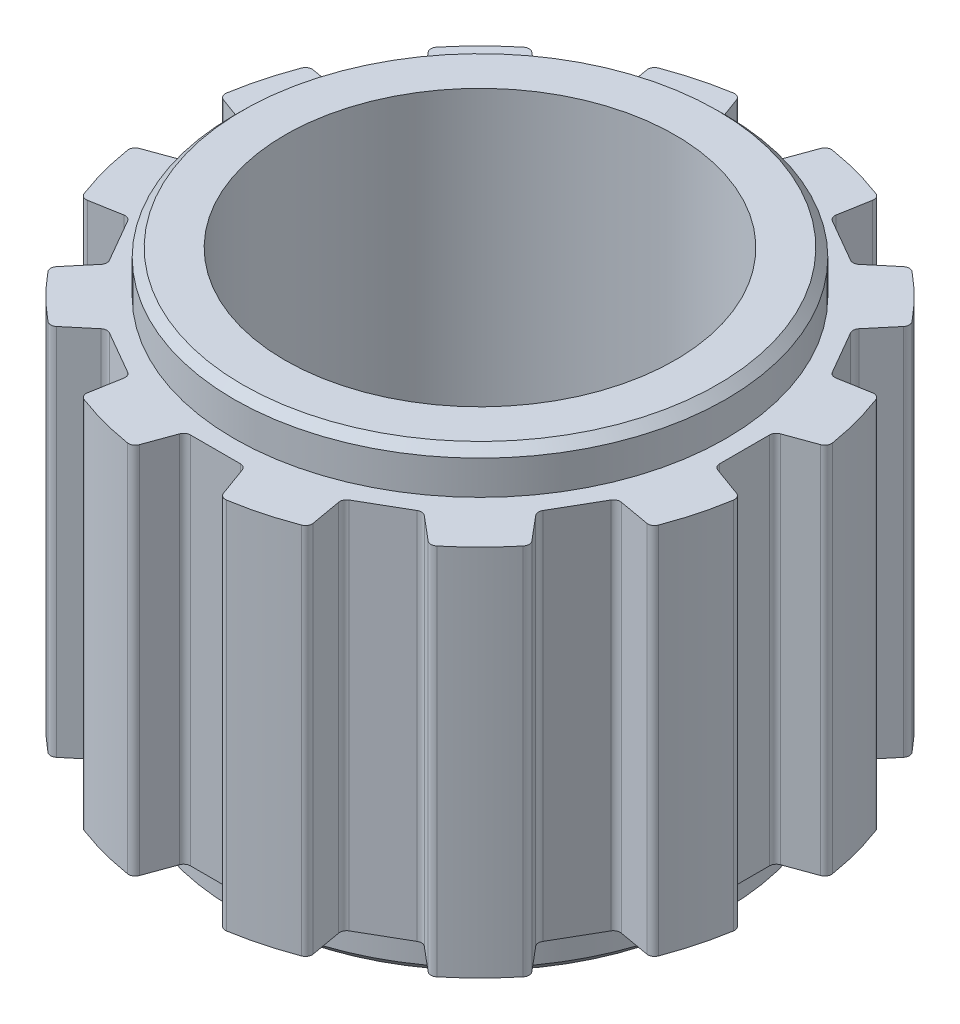
SolidWorks part; units mm, degrees
ref_plane "前视基准面" through (0, 0, 0) normal (0, 0, 1) x (1, 0, 0)
ref_plane "上视基准面" through (0, 0, 0) normal (0, 1, 0) x (1, 0, 0)
ref_plane "右视基准面" through (0, 0, 0) normal (1, 0, 0) x (0, 0, -1)
sketch "草图1" plane through (0, 0, 0) normal (0, 1, 0) x (1, 0, 0)
  line L0 (7.8, 13.51) -> (9.073, 12.775)
  line L1 (7.8, 13.51) -> (6.527, 14.245)
  line L2 (0, 15.6) -> (1.4699, 15.6)
  line L3 (0, 15.6) -> (-1.4699, 15.6)
  line L4 (-1.8458, 15.8632) -> (-2.4797, 17.6049)
  line L5 (1.8458, 15.8632) -> (2.4797, 17.6049)
  line L6 (6.3331, 14.6608) -> (6.655, 16.4862)
  line L7 (9.5301, 12.815) -> (10.95, 14.0065)
  line L8 (13.51, 7.8) -> (14.245, 6.527)
  line L9 (13.51, 7.8) -> (12.775, 9.073)
  line L10 (12.815, 9.5301) -> (14.0065, 10.95)
  line L11 (14.6608, 6.3331) -> (16.4862, 6.655)
  line L12 (15.6, 0) -> (15.6, -1.4699)
  line L13 (15.6, 0) -> (15.6, 1.4699)
  line L14 (15.8632, 1.8458) -> (17.6049, 2.4797)
  line L15 (15.8632, -1.8458) -> (17.6049, -2.4797)
  line L16 (13.51, -7.8) -> (12.775, -9.073)
  line L17 (13.51, -7.8) -> (14.245, -6.527)
  line L18 (14.6608, -6.3331) -> (16.4862, -6.655)
  line L19 (12.815, -9.5301) -> (14.0065, -10.95)
  line L20 (7.8, -13.51) -> (6.527, -14.245)
  line L21 (7.8, -13.51) -> (9.073, -12.775)
  line L22 (9.5301, -12.815) -> (10.95, -14.0065)
  line L23 (6.3331, -14.6608) -> (6.655, -16.4862)
  line L24 (0, -15.6) -> (-1.4699, -15.6)
  line L25 (0, -15.6) -> (1.4699, -15.6)
  line L26 (1.8458, -15.8632) -> (2.4797, -17.6049)
  line L27 (-1.8458, -15.8632) -> (-2.4797, -17.6049)
  line L28 (-7.8, -13.51) -> (-9.073, -12.775)
  line L29 (-7.8, -13.51) -> (-6.527, -14.245)
  line L30 (-6.3331, -14.6608) -> (-6.655, -16.4862)
  line L31 (-9.5301, -12.815) -> (-10.95, -14.0065)
  line L32 (-13.51, -7.8) -> (-14.245, -6.527)
  line L33 (-13.51, -7.8) -> (-12.775, -9.073)
  line L34 (-12.815, -9.5301) -> (-14.0065, -10.95)
  line L35 (-14.6608, -6.3331) -> (-16.4862, -6.655)
  line L36 (-15.6, 0) -> (-15.6, 1.4699)
  line L37 (-15.6, 0) -> (-15.6, -1.4699)
  line L38 (-15.8632, -1.8458) -> (-17.6049, -2.4797)
  line L39 (-15.8632, 1.8458) -> (-17.6049, 2.4797)
  line L40 (-13.51, 7.8) -> (-12.775, 9.073)
  line L41 (-13.51, 7.8) -> (-14.245, 6.527)
  line L42 (-14.6608, 6.3331) -> (-16.4862, 6.655)
  line L43 (-12.815, 9.5301) -> (-14.0065, 10.95)
  line L44 (-7.8, 13.51) -> (-6.527, 14.245)
  line L45 (-7.8, 13.51) -> (-9.073, 12.775)
  line L46 (-9.5301, 12.815) -> (-10.95, 14.0065)
  line L47 (-6.3331, 14.6608) -> (-6.655, 16.4862)
  circle A0 centre (0, 0) radius 19.1 construction
  arc A1 (-2.9201, 17.8629) -> (-6.4025, 16.9298) centre (0, 0) ccw
  arc A2 (-2.4797, 17.6049) -> (-2.9201, 17.8629) centre (-2.8556, 17.4681) ccw
  arc A3 (-1.4699, 15.6) -> (-1.8458, 15.8632) centre (-1.4699, 16) cw
  arc A4 (1.8458, 15.8632) -> (1.4699, 15.6) centre (1.4699, 16) cw
  arc A5 (2.9201, 17.8629) -> (2.4797, 17.6049) centre (2.8556, 17.4681) ccw
  arc A6 (6.655, 16.4862) -> (6.4025, 16.9298) centre (6.261, 16.5556) ccw
  arc A7 (6.527, 14.245) -> (6.3331, 14.6608) centre (6.727, 14.5914) cw
  arc A8 (9.5301, 12.815) -> (9.073, 12.775) centre (9.273, 13.1214) cw
  arc A9 (11.4604, 14.0096) -> (10.95, 14.0065) centre (11.2071, 13.7) ccw
  arc A10 (14.0065, 10.95) -> (14.0096, 11.4604) centre (13.7, 11.2071) ccw
  arc A11 (12.775, 9.073) -> (12.815, 9.5301) centre (13.1214, 9.273) cw
  arc A12 (14.6608, 6.3331) -> (14.245, 6.527) centre (14.5914, 6.727) cw
  arc A13 (16.9298, 6.4025) -> (16.4862, 6.655) centre (16.5556, 6.261) ccw
  arc A14 (17.6049, 2.4797) -> (17.8629, 2.9201) centre (17.4681, 2.8556) ccw
  arc A15 (15.6, 1.4699) -> (15.8632, 1.8458) centre (16, 1.4699) cw
  arc A16 (15.8632, -1.8458) -> (15.6, -1.4699) centre (16, -1.4699) cw
  arc A17 (17.8629, -2.9201) -> (17.6049, -2.4797) centre (17.4681, -2.8556) ccw
  arc A18 (16.4862, -6.655) -> (16.9298, -6.4025) centre (16.5556, -6.261) ccw
  arc A19 (14.245, -6.527) -> (14.6608, -6.3331) centre (14.5914, -6.727) cw
  arc A20 (12.815, -9.5301) -> (12.775, -9.073) centre (13.1214, -9.273) cw
  arc A21 (14.0096, -11.4604) -> (14.0065, -10.95) centre (13.7, -11.2071) ccw
  arc A22 (10.95, -14.0065) -> (11.4604, -14.0096) centre (11.2071, -13.7) ccw
  arc A23 (9.073, -12.775) -> (9.5301, -12.815) centre (9.273, -13.1214) cw
  arc A24 (6.3331, -14.6608) -> (6.527, -14.245) centre (6.727, -14.5914) cw
  arc A25 (6.4025, -16.9298) -> (6.655, -16.4862) centre (6.261, -16.5556) ccw
  arc A26 (2.4797, -17.6049) -> (2.9201, -17.8629) centre (2.8556, -17.4681) ccw
  arc A27 (1.4699, -15.6) -> (1.8458, -15.8632) centre (1.4699, -16) cw
  arc A28 (-1.8458, -15.8632) -> (-1.4699, -15.6) centre (-1.4699, -16) cw
  arc A29 (-2.9201, -17.8629) -> (-2.4797, -17.6049) centre (-2.8556, -17.4681) ccw
  arc A30 (-6.655, -16.4862) -> (-6.4025, -16.9298) centre (-6.261, -16.5556) ccw
  arc A31 (-6.527, -14.245) -> (-6.3331, -14.6608) centre (-6.727, -14.5914) cw
  arc A32 (-9.5301, -12.815) -> (-9.073, -12.775) centre (-9.273, -13.1214) cw
  arc A33 (-11.4604, -14.0096) -> (-10.95, -14.0065) centre (-11.2071, -13.7) ccw
  arc A34 (-14.0065, -10.95) -> (-14.0096, -11.4604) centre (-13.7, -11.2071) ccw
  arc A35 (-12.775, -9.073) -> (-12.815, -9.5301) centre (-13.1214, -9.273) cw
  arc A36 (-14.6608, -6.3331) -> (-14.245, -6.527) centre (-14.5914, -6.727) cw
  arc A37 (-16.9298, -6.4025) -> (-16.4862, -6.655) centre (-16.5556, -6.261) ccw
  arc A38 (-17.6049, -2.4797) -> (-17.8629, -2.9201) centre (-17.4681, -2.8556) ccw
  arc A39 (-15.6, -1.4699) -> (-15.8632, -1.8458) centre (-16, -1.4699) cw
  arc A40 (-15.8632, 1.8458) -> (-15.6, 1.4699) centre (-16, 1.4699) cw
  arc A41 (-17.8629, 2.9201) -> (-17.6049, 2.4797) centre (-17.4681, 2.8556) ccw
  arc A42 (-16.4862, 6.655) -> (-16.9298, 6.4025) centre (-16.5556, 6.261) ccw
  arc A43 (-14.245, 6.527) -> (-14.6608, 6.3331) centre (-14.5914, 6.727) cw
  arc A44 (-12.815, 9.5301) -> (-12.775, 9.073) centre (-13.1214, 9.273) cw
  arc A45 (-14.0096, 11.4604) -> (-14.0065, 10.95) centre (-13.7, 11.2071) ccw
  arc A46 (-10.95, 14.0065) -> (-11.4604, 14.0096) centre (-11.2071, 13.7) ccw
  arc A47 (-9.073, 12.775) -> (-9.5301, 12.815) centre (-9.273, 13.1214) cw
  arc A48 (-6.3331, 14.6608) -> (-6.527, 14.245) centre (-6.727, 14.5914) cw
  arc A49 (-6.4025, 16.9298) -> (-6.655, 16.4862) centre (-6.261, 16.5556) ccw
  arc A50 (-11.4604, 14.0096) -> (-14.0096, 11.4604) centre (0, 0) ccw
  arc A51 (-16.9298, 6.4025) -> (-17.8629, 2.9201) centre (0, 0) ccw
  arc A52 (-17.8629, -2.9201) -> (-16.9298, -6.4025) centre (0, 0) ccw
  arc A53 (-14.0096, -11.4604) -> (-11.4604, -14.0096) centre (0, 0) ccw
  arc A54 (-6.4025, -16.9298) -> (-2.9201, -17.8629) centre (0, 0) ccw
  arc A55 (2.9201, -17.8629) -> (6.4025, -16.9298) centre (0, 0) ccw
  arc A56 (11.4604, -14.0096) -> (14.0096, -11.4604) centre (0, 0) ccw
  arc A57 (16.9298, -6.4025) -> (17.8629, -2.9201) centre (0, 0) ccw
  arc A58 (17.8629, 2.9201) -> (16.9298, 6.4025) centre (0, 0) ccw
  arc A59 (14.0096, 11.4604) -> (11.4604, 14.0096) centre (0, 0) ccw
  arc A60 (6.4025, 16.9298) -> (2.9201, 17.8629) centre (0, 0) ccw
  circle A61 centre (0, 0) radius 11.5
  point P15 (-1.75, 15.6)
  point P18 (1.75, 15.6)
  dimension "D4" = 0.4
  dimension "D2" = 1.75
  dimension "D3" = 1.75
extrude "拉伸1" add sketch "草图1" along normal blind 27
sketch "草图2" plane through (0, 27, 0) normal (0, 1, 0) x (-1, 0, 0)
  circle A0 centre (0, 0) radius 14.5
  circle A1 centre (0, 0) radius 18.1
extrude "切除-拉伸1" cut sketch "草图2" against normal blind 2.5
sketch "草图3" plane through (0, 0, 0) normal (0, -1, 0) x (1, 0, 0)
  circle A0 centre (0, 0) radius 14.5
  circle A1 centre (0, 0) radius 18.1
extrude "切除-拉伸2" cut sketch "草图3" against normal blind 2.5
chamfer "倒角1" distance 0.5 angle 45 2 edges at (0, 27, 14.5) (0, 0, -14.5)
